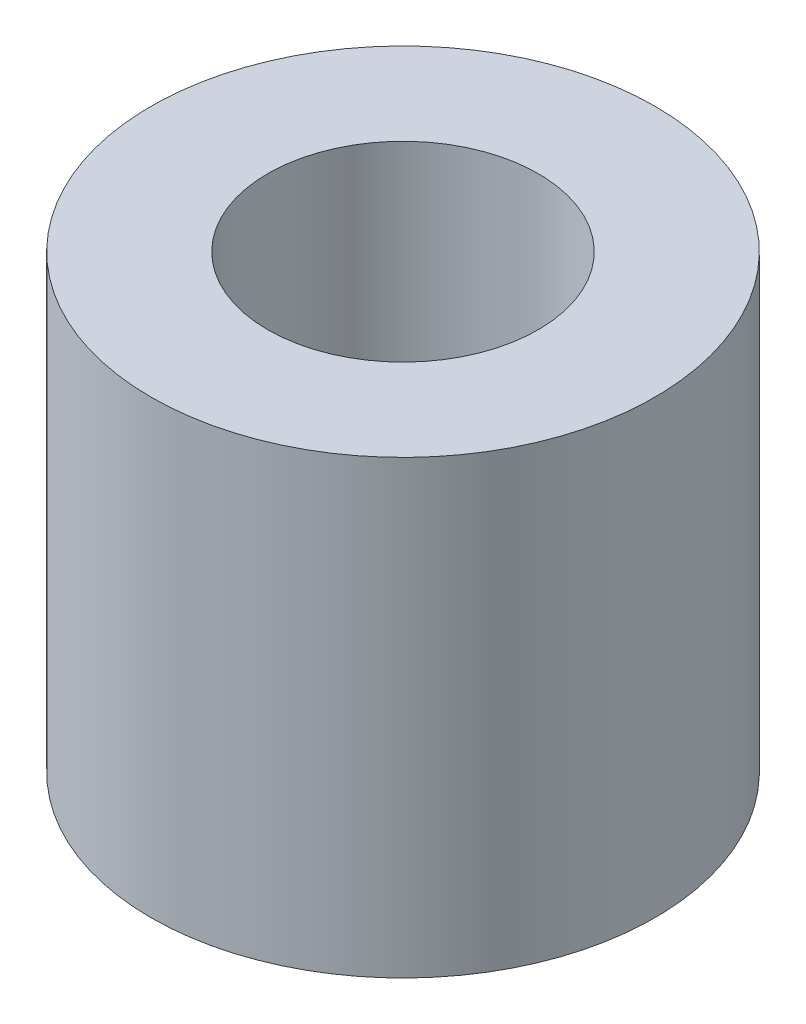
from build123d import *

# Parameters (mm, degrees)
SKETCH1_R              = 9.5
SKETCH1_R_2            = 4.5
BOSS_EXTRUDE1_DEPTH    = 17
M12_TAPPED_HOLE1_D     = 10.2
M12_TAPPED_HOLE1_DEPTH = 32.75
M12_TAPPED_HOLE1_TIP   = 3.064389157


with BuildPart() as part:
    # Sketch1 → Boss-Extrude1 (new body)
    with BuildSketch(Plane(origin=(0, 0, 0), x_dir=(1, 0, 0), z_dir=(0, 1, 0))):
        with Locations(Location((0, 0, 0), (0, 0, 270))):
            Circle(SKETCH1_R)
        with Locations(Location((0, 0, 0), (0, 0, 270))):
            Circle(SKETCH1_R_2, mode=Mode.SUBTRACT)
    extrude(amount=BOSS_EXTRUDE1_DEPTH)

    # M12 Tapped Hole1
    with Locations(Plane(origin=(0, 17, 0), x_dir=(1, 0, 0), z_dir=(0, 1, 0))):
        with Locations((0, 0)):
            Hole(M12_TAPPED_HOLE1_D / 2, depth=M12_TAPPED_HOLE1_DEPTH)
            with Locations((0, 0, -(M12_TAPPED_HOLE1_DEPTH + M12_TAPPED_HOLE1_TIP / 2))):  # 118° drill point
                Cone(0, M12_TAPPED_HOLE1_D / 2, M12_TAPPED_HOLE1_TIP, mode=Mode.SUBTRACT)


solid = part.part
